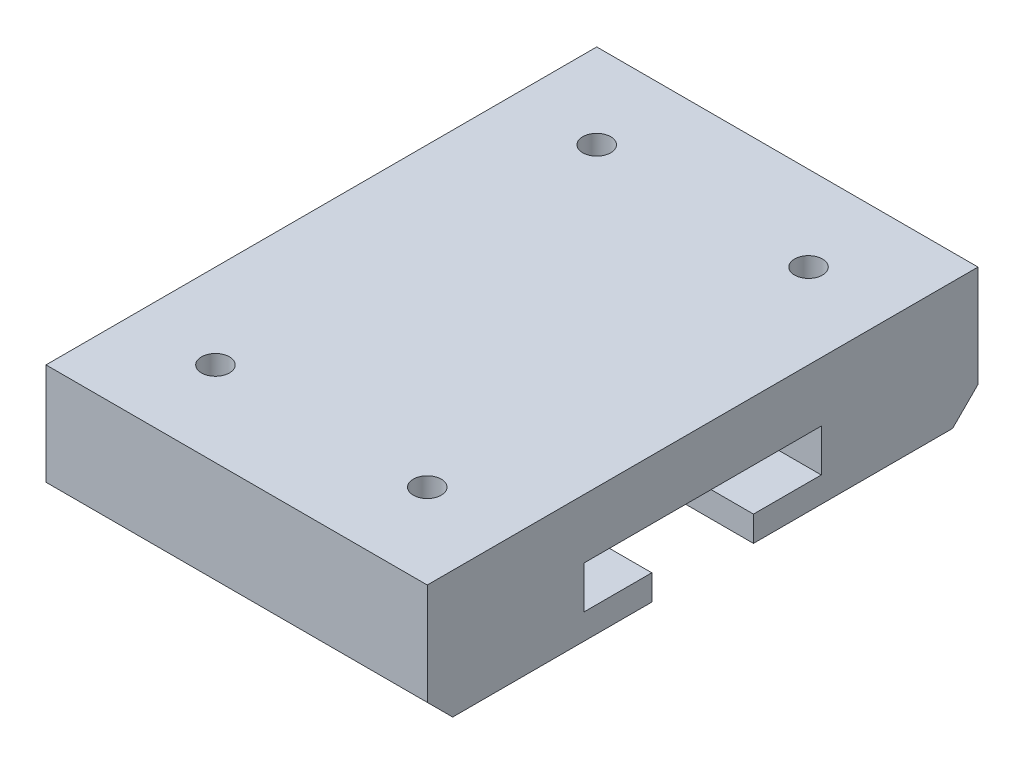
from build123d import *

# Parameters (mm, degrees)
BOSS_EXTRUDE1_DEPTH = 22.5
CHAMFER1_SIZE       = 3
M4_TAPPED_HOLE1_D   = 3.3


with BuildPart() as part:
    # Sketch2 → Boss-Extrude1 (new, symmetric)
    with BuildSketch(Plane(origin=(0, 0, 0), x_dir=(0, 0, -1), z_dir=(1, 0, 0))):
        Polygon((67.5, 0), (132.5, 0), (132.5, -15), (106, -15), (106, -12), (114, -12), (114, -7), (86, -7), (86, -12), (94, -12), (94, -15), (67.5, -15), align=None)
    extrude(amount=BOSS_EXTRUDE1_DEPTH, both=True)

    # Chamfer1
    chamfer1_edges = [part.edges().sort_by_distance(p)[0] for p in [
        (0, -15, -132.5),
        (0, -15, -67.5),
    ]]
    chamfer(chamfer1_edges, length=CHAMFER1_SIZE)

    # M4 Tapped Hole1 (through all)
    with Locations(Plane(origin=(0, 0, 0), x_dir=(1, 0, 0), z_dir=(0, 1, 0))):
        with Locations((-12.5, 122.5), (12.5, 122.5), (-12.5, 77.5), (12.5, 77.5)):
            Hole(M4_TAPPED_HOLE1_D / 2)


solid = part.part
